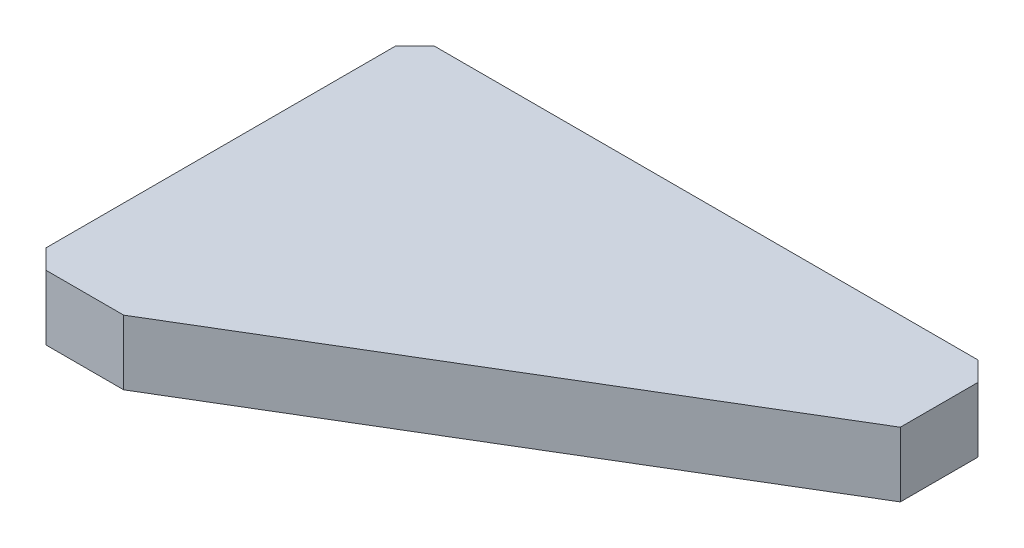
SolidWorks part; units mm, degrees
material "A6061 T6"
ref_plane "前视基准面" through (0, 0, 0) normal (0, 0, 1) x (1, 0, 0)
ref_plane "上视基准面" through (0, 0, 0) normal (0, 1, 0) x (1, 0, 0)
ref_plane "右视基准面" through (0, 0, 0) normal (1, 0, 0) x (0, 0, -1)
sketch "草图1" plane through (0, 0, 0) normal (0, 1, 0) x (1, 0, 0)
  line L1 (-45, 30) -> (45, 30)
  line L2 (-45, 30) -> (-45, -30)
  line L3 (-45, -30) -> (45, -30)
  line L4 (45, 30) -> (45, -30)
  line L5 (-45, 30) -> (45, -30) construction
  line L6 (-45, -30) -> (45, 30) construction
  point P0 (0, 0)
  dimension "D1" = 60
  dimension "D2" = 90
extrude "凸台-拉伸1" add sketch "草图1" along normal blind 10
sketch "草图2" plane through (0, 10, 0) normal (0, 1, 0) x (1, 0, 0)
  line L0 (45, 15) -> (-30, -30)
  line L1 (45, -30) -> (45, 30) construction
  line L2 (-45, -30) -> (45, -30) construction
  line L3 (-30, -30) -> (45, -30)
  line L4 (45, -30) -> (45, 15)
  line L5 (-45, 30) -> (-45, -30) construction
  line L6 (45, 30) -> (-45, 30) construction
  dimension "D1" = 15
  dimension "D2" = 15
extrude "切除-拉伸1" cut sketch "草图2" against normal blind 15
chamfer "倒角1" distance 3 angle 45 3 edges at (45, 5, -30) (-45, 5, 30) (-45, 5, -30)
hole_wizard "M5 螺纹孔1" positions "草图3" profile "草图4" tap size "M5" standard "GB"
sketch "草图3" plane through (-45, 0, 0) normal (-1, 0, 0) x (0, 0, 1)
  line L0 (-27, 10) -> (27, 10) construction
  line L1 (-30, 0) -> (-30, 10) construction
  line L2 (30, 10) -> (30, 0) construction
  point P0 (-15, 5)
  point P2 (15, 5)
  dimension "D1" = 5
  dimension "D2" = 15
  dimension "D3" = 15
sketch "草图4" plane through (-45, 5, -15) normal (0, 1, 0) x (0, 0, 1)
  line L0 (0, 0) -> (0, 13.6618)
  line L1 (0, 13.6618) -> (2.1, 12.4)
  line L2 (2.1, 12.4) -> (2.1, 0)
  line L5 (2.1, 0) -> (0, 0)
  line L10 (0, 13.6618) -> (-2.1, 12.4) construction
  line L11 (0, -6.35) -> (0, 107.95) construction
  dimension "螺纹孔钻头直径" = 4.2
  dimension "螺纹孔钻头深度" = 12.4
  dimension "导头角度" = 118
cosmetic thread "孔螺蚊线1" parameters "D1"=10, "D2"=5
cosmetic thread "孔螺蚊线2" parameters "D1"=10, "D2"=5
hole_wizard "M5 螺纹孔2" positions "草图5" profile "草图6" tap size "M5" standard "GB"
sketch "草图5" plane through (0, 0, -30) normal (0, 0, -1) x (-1, 0, 0)
  line L0 (-42, 0) -> (42, 0) construction
  line L1 (45, 10) -> (45, 0) construction
  line L2 (-45, 0) -> (-45, 10) construction
  point P0 (30, 5)
  point P2 (0, 5)
  point P4 (-30, 5)
  dimension "D1" = 5
  dimension "D2" = 15
  dimension "D3" = 15
  dimension "D4" = 30
sketch "草图6" plane through (-30, 5, -30) normal (1, 0, 0) x (0, 1, 0)
  line L0 (0, 0) -> (0, 13.6618)
  line L1 (0, 13.6618) -> (2.1, 12.4)
  line L2 (2.1, 12.4) -> (2.1, 0)
  line L5 (2.1, 0) -> (0, 0)
  line L10 (0, 13.6618) -> (-2.1, 12.4) construction
  line L11 (0, -6.35) -> (0, 107.95) construction
  dimension "螺纹孔钻头直径" = 4.2
  dimension "螺纹孔钻头深度" = 12.4
  dimension "导头角度" = 118
cosmetic thread "孔螺蚊线3"
cosmetic thread "孔螺蚊线4"
cosmetic thread "孔螺蚊线5"
